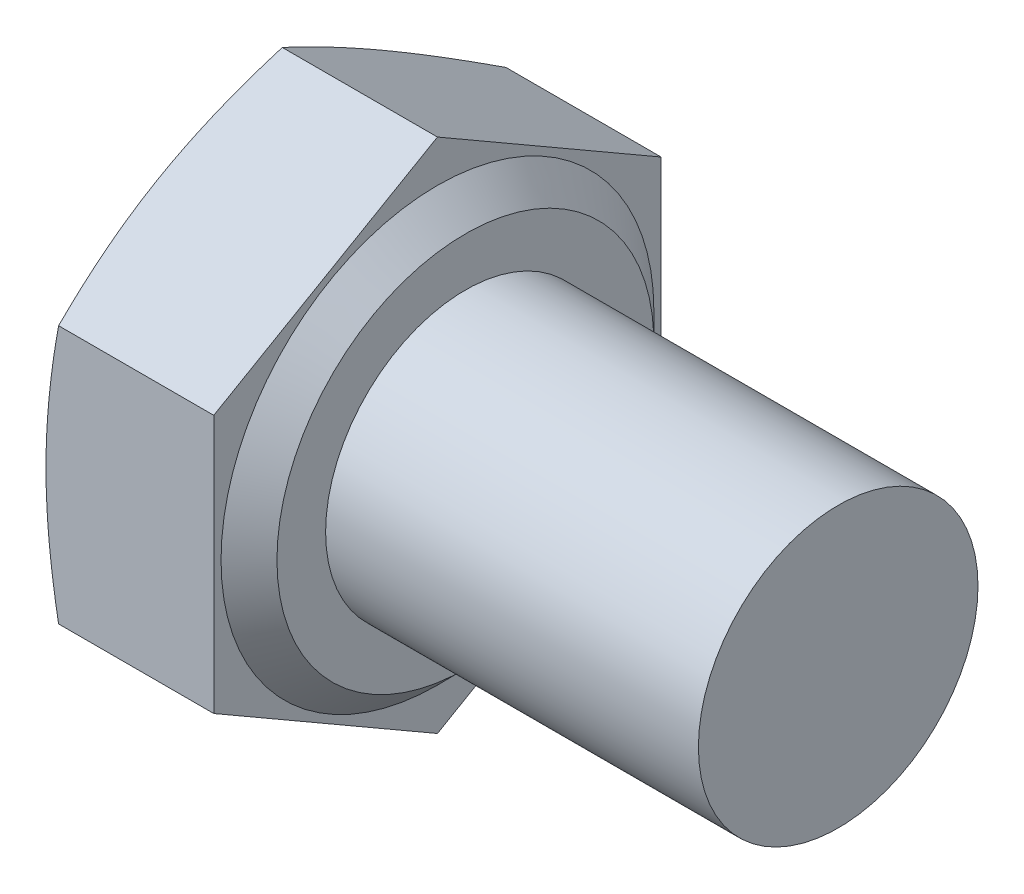
SolidWorks part; units mm, degrees
ref_plane "Front" through (0, 0, 0) normal (0, 0, 1) x (1, 0, 0)
ref_plane "Top" through (0, 0, 0) normal (0, 1, 0) x (1, 0, 0)
ref_plane "Right" through (0, 0, 0) normal (1, 0, 0) x (0, 0, -1)
sketch "Sketch2" plane through (0, 0, 0) normal (1, 0, 0) x (0, 0, -1)
  line L1 (0, -4.6188) -> (4, -2.3094)
  line L2 (4, -2.3094) -> (4, 2.3094)
  line L3 (4, 2.3094) -> (0, 4.6188)
  line L4 (0, 4.6188) -> (-4, 2.3094)
  line L5 (-4, 2.3094) -> (-4, -2.3094)
  line L6 (-4, -2.3094) -> (0, -4.6188)
  circle A0 centre (0, 0) radius 4 construction
extrude "BaseHead" add sketch "Sketch2" along normal blind 3.5
sketch "Sketch3" plane through (0, 0, 0) normal (0, 0, 1) x (1, 0, 0)
  line L0 (3.5, 4.6188) -> (3.5, 3.37)
  line L2 (3.5, 3.37) -> (3, 3.87)
  line L3 (3, 3.87) -> (3, 4.6188)
  line L5 (3, 4.6188) -> (3.5, 4.6188)
  line L6 (-0.9571, 0) -> (7.6478, 0) construction
  line L7 (3.5, 4.6188) -> (0, 4.6188) construction
  dimension "D1" = 45
  dimension "c" = 0.5
  dimension "dw" = 6.74
revolve "BearingFace" cut sketch "Sketch3" angle 360 about L6
sketch "Sketch4" plane through (0, 0, 0) normal (0, 0, 1) x (1, 0, 0)
  line L0 (-0.4935, 0) -> (3.5626, 0) construction
  line L2 (0, 4.6188) -> (0.2252, 4.6188)
  line L4 (0.2252, 4.6188) -> (0, 4)
  line L6 (0, 4) -> (0, 4.6188)
  line L7 (3, 4.6188) -> (0, 4.6188) construction
revolve "HeadChamfer" cut sketch "Sketch4" angle 360 about L0
sketch "Sketch5" plane through (3.5, 0, 0) normal (1, 0, 0) x (0, 0, -1)
  circle A0 centre (0, 0) radius 2.5
extrude "BaseBody" add sketch "Sketch5" along normal blind 10
cosmetic thread "ThreadCosmetic1" [suppressed] parameters "D2"=4.134
chamfer "Chamfer1" distance 0.25 angle 45 1 edges at (13.5, 0, -2.5)
fillet "HeadFillet" [suppressed] radius 0.2
sketch "Sketch6" plane through (0, 0, 0) normal (0, 0, 1) x (1, 0, 0)
  line L0 (3.5, 2.933) -> (3.933, 2.933)
  line L1 (3.933, 2.933) -> (3.933, 2.5)
  line L2 (3.933, 2.5) -> (3.7165, 2.125)
  line L3 (3.7165, 2.125) -> (3.5, 2.5)
  line L4 (3.5, 2.5) -> (3.5, 2.933)
  line L5 (3.5, -3.37) -> (3.5, 3.37) construction
  line L6 (13.25, 2.5) -> (3.5, 2.5) construction
revolve "Cut-Revolve10" [suppressed] cut sketch "Sketch6" angle 360
pattern_linear "LPattern10" [suppressed] count 19
scale "Scale1" scale about centroid uniform scaling yes scale factor 0.6
sketch "Sketch1" plane through (10.1697, 0, 0) normal (1, 0, 0) x (0, 0, -1)
  circle A0 centre (0, 0) radius 1.9182
extrude "Cut-Extrude1" cut sketch "Sketch1" against normal blind 2
equation "\"D2@Sketch4\" = \"s@Sketch2\""
equation "\"D1@Chamfer1\" = 0.05 * \"d@Sketch5\""
equation "\"D1@Sketch6\" =  ( \"d@Sketch5\" - \"D2@ThreadCosmetic1\" )  / 2"
equation "\"pitch@LPattern10\" = 1.2 * \"D1@Sketch6\""
equation "\"D1@LPattern10\" = (  \"l@BaseBody\"-\"D1@Chamfer1\" )  / \"pitch@LPattern10\""
